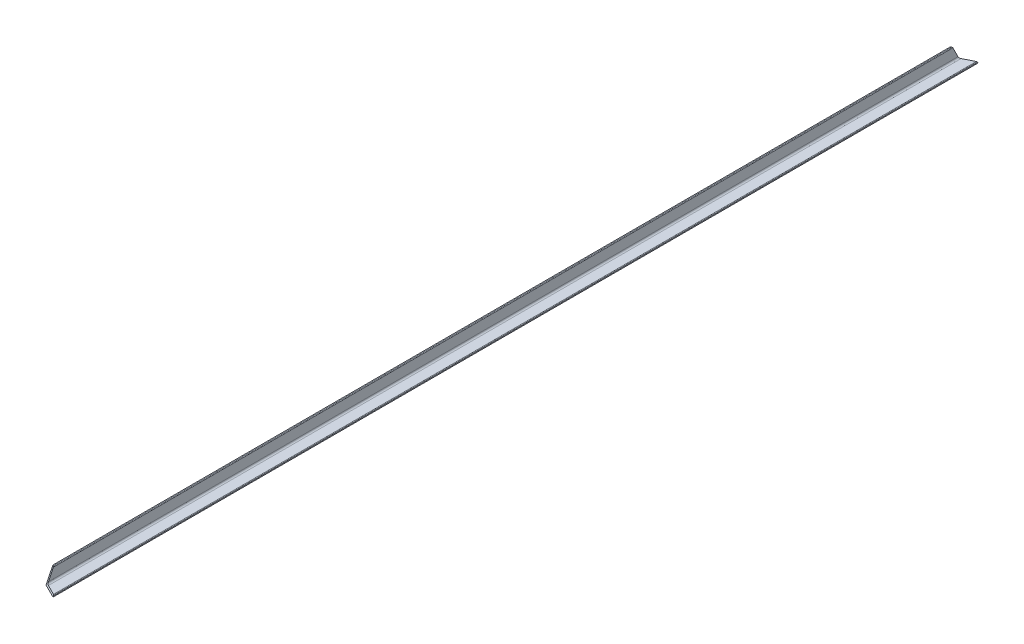
from build123d import *

# Parameters (mm, degrees)
BOSS_EXTRUDE1_DEPTH     = 4645
CUT_EXTRUDE4_DEPTH      = 4647.054777981
CUT_EXTRUDE4_DEPTH_BACK = 10


with BuildPart() as part:
    # Sketch1 → Boss-Extrude1 (new body)
    with BuildSketch(Plane.XY):
        with BuildLine():
            Line((0, 70), (0, 0))
            Line((0, 0), (70, 0))
            Line((70, 0), (70, 5))
            ThreePointArc((70, 5), (69.121320344, 7.121320344), (67, 8))
            Line((67, 8), (16, 8))
            ThreePointArc((16, 8), (10.343145751, 10.343145751), (8, 16))
            Line((8, 16), (8, 67))
            ThreePointArc((8, 67), (7.121320344, 69.121320344), (5, 70))
            Line((5, 70), (0, 70))
        make_face()
    extrude(amount=BOSS_EXTRUDE1_DEPTH)

    # Sketch3 → Cut-Extrude4 (cut, two sides: drawn at the far end of the back side and taken through both)
    with BuildSketch(Plane(origin=(0, 0, 0), x_dir=(0, 0, -1), z_dir=(0.7071067811865488, 0.7071067811865464, 0)).offset(-CUT_EXTRUDE4_DEPTH_BACK)):
        Polygon((0, -49.497474683), (-69.317009791, 49.497474683), (0, 49.497474683), align=None)
        Polygon((-4645, -49.497474683), (-4645, 49.497474683), (-4575.682990209, 49.497474683), align=None)
    extrude(amount=CUT_EXTRUDE4_DEPTH + CUT_EXTRUDE4_DEPTH_BACK, mode=Mode.SUBTRACT)


solid = part.part
